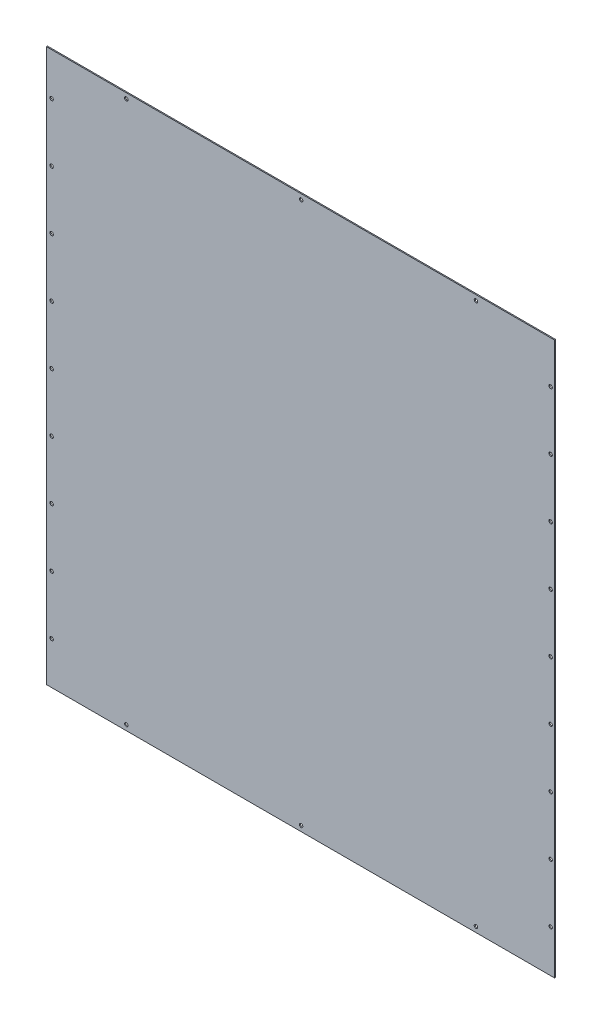
SolidWorks part; units mm, degrees
material "304"
ref_plane "前视基准面" through (0, 0, 0) normal (0, 0, 1) x (1, 0, 0)
ref_plane "上视基准面" through (0, 0, 0) normal (0, 1, 0) x (1, 0, 0)
ref_plane "右视基准面" through (0, 0, 0) normal (1, 0, 0) x (0, 0, -1)
sketch "草图1" plane through (0, 0, 0) normal (0, 0, 1) x (1, 0, 0)
  line L0 (0, 0) -> (451.2544, 0) construction
  line L1 (-481, 521.5) -> (481, 521.5)
  line L2 (-481, 521.5) -> (-481, -521.5)
  line L3 (-481, -521.5) -> (481, -521.5)
  line L4 (481, 521.5) -> (481, -521.5)
  line L5 (-481, 521.5) -> (481, -521.5) construction
  line L6 (-481, -521.5) -> (481, 521.5) construction
  line L7 (0, 0) -> (0, 412.8629) construction
  circle A0 centre (-471, 0) radius 3.25
  circle A1 centre (-471, -110.375) radius 3.25
  circle A2 centre (-471, -220.75) radius 3.25
  circle A3 centre (-471, -331.125) radius 3.25
  circle A4 centre (-471, -441.5) radius 3.25
  circle A34 centre (0, -511.5) radius 3.25
  circle A35 centre (0, 511.5) radius 3.25
  circle A36 centre (-471, 441.5) radius 3.25
  circle A37 centre (-471, 331.125) radius 3.25
  circle A38 centre (-471, 220.75) radius 3.25
  circle A39 centre (-471, 110.375) radius 3.25
  circle A40 centre (471, 110.375) radius 3.25
  circle A41 centre (471, 220.75) radius 3.25
  circle A42 centre (471, 331.125) radius 3.25
  circle A43 centre (471, 441.5) radius 3.25
  circle A44 centre (471, -441.5) radius 3.25
  circle A45 centre (471, -331.125) radius 3.25
  circle A46 centre (471, -220.75) radius 3.25
  circle A47 centre (471, -110.375) radius 3.25
  circle A48 centre (471, 0) radius 3.25
  circle A49 centre (330, -511.5) radius 3.25
  circle A50 centre (-330, -511.5) radius 3.25
  circle A51 centre (-330, 511.5) radius 3.25
  circle A52 centre (330, 511.5) radius 3.25
  point P0 (0, 0)
  dimension "D3" = 6.5
  dimension "D8" = 660
  dimension "D1" = 962
  dimension "D2" = 1043
  dimension "D4" = 10
  dimension "D6" = 10
  dimension "D7" = 80
  dimension "D5" = 5
extrude "凸台-拉伸1" add sketch "草图1" along normal blind 2
sketch "草图2" plane through (0, -521.5, 0) normal (0, -1, 0) x (1, 0, 0)
  line L0 (-481, 2) -> (481, 2) construction
  line L1 (481, 0) -> (478.5, 0)
  line L2 (481, 0) -> (481, 2)
  line L3 (481, 2) -> (478.5, 2)
  line L4 (478.5, 0) -> (478.5, 2)
  line L5 (481, 0) -> (478.5, 2) construction
  line L6 (481, 2) -> (478.5, 0) construction
  point P4 (479.75, 1)
  dimension "D1" = 2.5
extrude "切除-拉伸1" cut sketch "草图2" against normal through all
